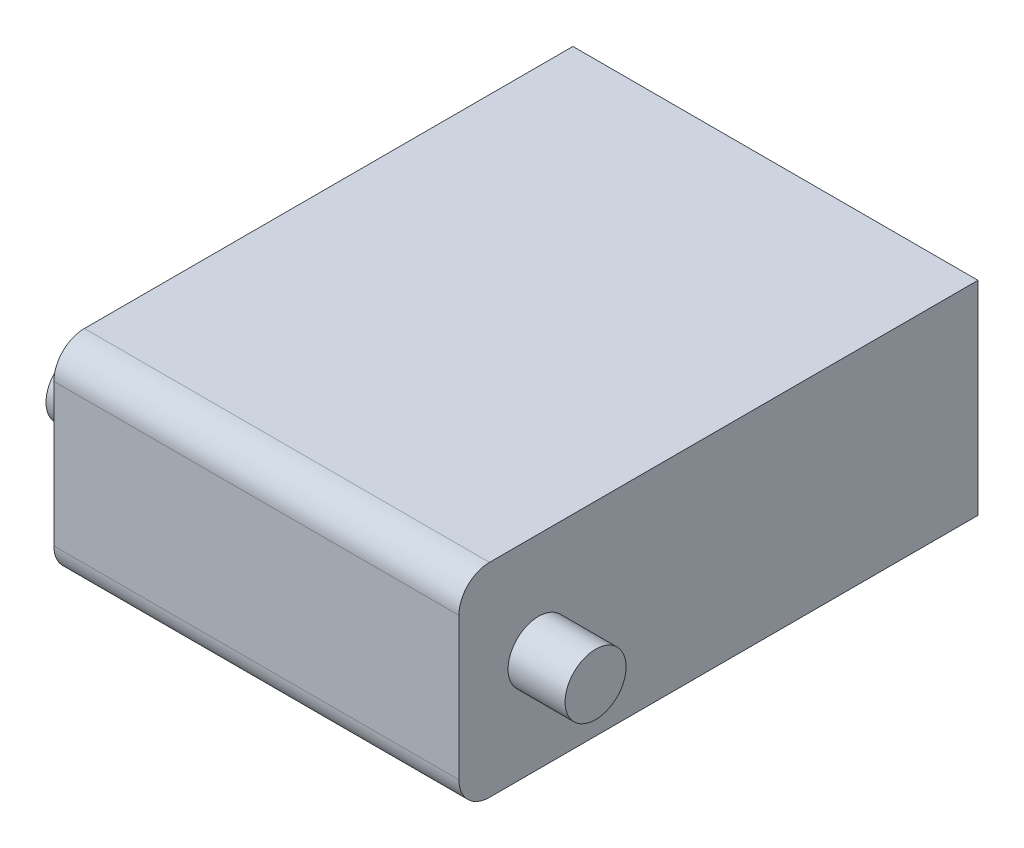
SolidWorks part; units mm, degrees
ref_plane "Front Plane" through (0, 0, 0) normal (0, 0, 1) x (1, 0, 0)
ref_plane "Top Plane" through (0, 0, 0) normal (0, 1, 0) x (1, 0, 0)
ref_plane "Right Plane" through (0, 0, 0) normal (1, 0, 0) x (0, 0, -1)
other "Configuration Table"
sketch "Sketch1" plane through (0, 0, 0) normal (0, 0, 1) x (1, 0, 0)
  line L1 (-19.9, 10) -> (19.9, 10)
  line L2 (-19.9, 10) -> (-19.9, -10)
  line L3 (-19.9, -10) -> (19.9, -10)
  line L4 (19.9, 10) -> (19.9, -10)
  line L5 (-19.9, 10) -> (19.9, -10) construction
  line L6 (-19.9, -10) -> (19.9, 10) construction
  point P0 (0, 0)
  dimension "D1" = 39.8
  dimension "D2" = 20
extrude "Boss-Extrude1" add sketch "Sketch1" along normal blind 51
sketch "Sketch2" plane through (0, 0, 0) normal (1, 0, 0) x (0, 0, -1)
  circle A0 centre (-43.1736, 0) radius 3
  dimension "D1" = 6
extrude "Boss-Extrude2" add sketch "Sketch2" along normal mid plane 51
sketch "Sketch6" plane through (0, 0, 0) normal (0, 0, -1) x (-1, 0, 0)
  line L0 (-19.9, 0) -> (19.9, 0) construction
  line L1 (-19.9, -10) -> (-19.9, 10) construction
  line L2 (19.9, -3) -> (19.9, 3) construction
  line L3 (0, 0) -> (0, 8.0504) construction
  line L4 (12.5, 0) -> (12.5, 6.9308) construction
  line L5 (-12.5, 0) -> (-12.5, 5.6513) construction
  dimension "D1" = 25
  dimension "D2" = 12.5
hole_wizard "M3 Tapped Hole1" positions "3DSketch1" profile "Sketch8" tap size "M3" standard "GB"
sketch3d "3DSketch1"
  line L0 (19.9, 0, 0) -> (-19.9, 0, 0) construction
  point P0 (12.5, 0, 0)
  point P3 (0, 0, 0)
  point P6 (-12.5, 0, 0)
  point P9 (-0.1209, 0, 0)
sketch "Sketch8" plane through (12.5, 0, 0) normal (1, 0, 0) x (0, 1, 0)
  line L0 (0, 0) -> (0, 8.2511)
  line L1 (0, 8.2511) -> (1.25, 7.5)
  line L2 (1.25, 7.5) -> (1.25, 0)
  line L5 (1.25, 0) -> (0, 0)
  line L10 (0, 8.2511) -> (-1.25, 7.5) construction
  line L11 (0, -6.35) -> (0, 107.95) construction
  dimension "螺纹孔钻头直径" = 2.5
  dimension "螺纹孔钻头深度" = 7.5
  dimension "导头角度" = 118
cosmetic thread "Cosmetic thread 1" parameters "D1"=6, "D2"=3
cosmetic thread "Cosmetic thread 2" parameters "D1"=6, "D2"=3
cosmetic thread "Cosmetic thread 3" parameters "D1"=6, "D2"=3
cosmetic thread "Cosmetic thread 4" parameters "D1"=6, "D2"=3
fillet "Fillet1" radius 3 2 edges at (0, -10, 51) (0, 10, 51)
